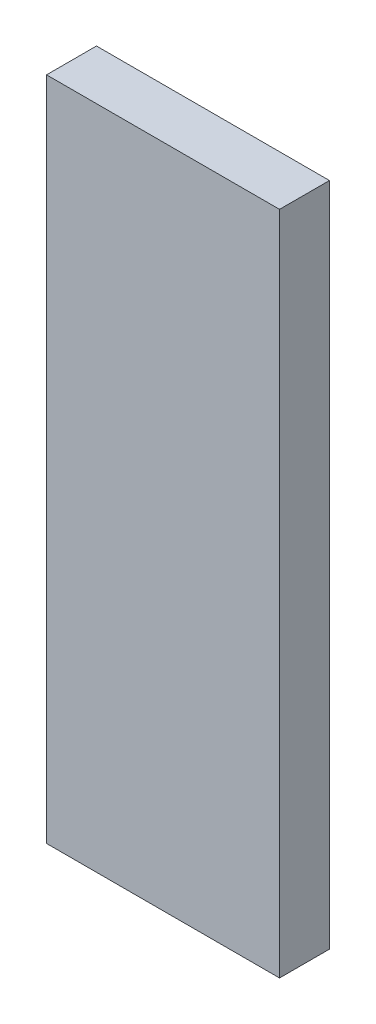
from build123d import *

# Parameters (mm, degrees)
SKETCH1_W           = 70
SKETCH1_H           = 200
BOSS_EXTRUDE1_DEPTH = 7.5


with BuildPart() as part:
    # Sketch1 → Boss-Extrude1 (new, symmetric)
    with BuildSketch(Plane.XY):
        Rectangle(SKETCH1_W, SKETCH1_H)
    extrude(amount=BOSS_EXTRUDE1_DEPTH, both=True)


solid = part.part
